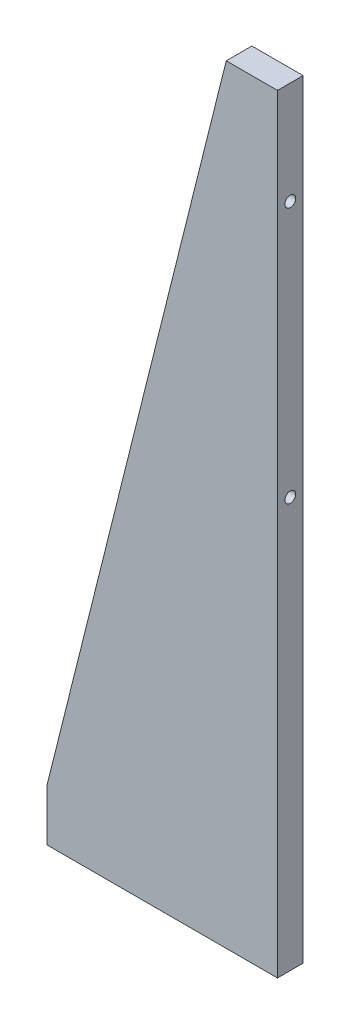
SolidWorks part; units mm, degrees
ref_plane "前视基准面" through (0, 0, 0) normal (0, 0, 1) x (1, 0, 0)
ref_plane "上视基准面" through (0, 0, 0) normal (0, 1, 0) x (1, 0, 0)
ref_plane "右视基准面" through (0, 0, 0) normal (1, 0, 0) x (0, 0, -1)
sketch "草图1" plane through (0, 0, 0) normal (0, 0, 1) x (1, 0, 0)
  line L1 (45, -150) -> (-45, -150)
  line L2 (45, -150) -> (45, 150)
  line L3 (45, 150) -> (-45, 150)
  line L4 (-45, -150) -> (-45, 150)
  line L5 (45, -150) -> (-45, 150) construction
  line L6 (45, 150) -> (-45, -150) construction
  point P0 (0, 0)
  dimension "D1" = 300
  dimension "D2" = 90
extrude "凸台-拉伸1" add sketch "草图1" along normal blind 10
sketch "草图2" plane through (0, 0, 10) normal (0, 0, 1) x (1, 0, 0)
  line L0 (25, 150) -> (-45, 150)
  line L1 (45, 150) -> (-45, 150) construction
  line L2 (-45, 150) -> (-45, -130)
  line L3 (-45, 150) -> (-45, -150) construction
  line L4 (-45, -130) -> (25, 150)
  line L5 (45, -150) -> (45, 150) construction
  line L6 (-45, -150) -> (45, -150) construction
  dimension "D1" = 20
  dimension "D2" = 20
extrude "切除-拉伸1" cut sketch "草图2" against normal up to next
hole_wizard "M5 螺纹孔1" positions "草图3" profile "草图5" tap size "M5" standard "GB"
sketch "草图3" plane through (0, -150, 0) normal (0, -1, 0) x (-1, 0, 0)
  line L0 (-45, -5) -> (-25, -5) construction
  line L1 (-45, -10) -> (-45, 0) construction
  line L2 (-25, -5) -> (25, -5) construction
  line L5 (0, -5) -> (0, 0) construction
  line L6 (45, 0) -> (-45, 0) construction
  point P0 (-25, -5)
  point P2 (25, -5)
  dimension "D1" = 50
sketch "草图5" plane through (25, -150, 5) normal (1, 0, 0) x (0, 0, -1)
  line L0 (0, 0) -> (0, 15.6618)
  line L1 (0, 15.6618) -> (2.1, 14.4)
  line L2 (2.1, 14.4) -> (2.1, 0)
  line L5 (2.1, 0) -> (0, 0)
  line L10 (0, 15.6618) -> (-2.1, 14.4) construction
  line L11 (0, -6.35) -> (0, 107.95) construction
  dimension "螺纹孔钻头直径" = 4.2
  dimension "螺纹孔钻头深度" = 14.4
  dimension "导头角度" = 118
cosmetic thread "孔螺蚊线1" parameters "D1"=12, "D2"=5
cosmetic thread "孔螺蚊线2" parameters "D1"=12, "D2"=5
hole_wizard "M5 螺纹孔2" positions "草图6" profile "草图7" tap size "M5" standard "GB"
sketch "草图6" plane through (45, 0, 0) normal (1, 0, 0) x (0, 0, -1)
  line L0 (-5, 150) -> (-5, 110) construction
  line L1 (-10, 150) -> (0, 150) construction
  line L2 (-5, 110) -> (-5, 10) construction
  point P0 (-5, 110)
  point P2 (-5, 10)
  dimension "D1" = 40
  dimension "D2" = 100
sketch "草图7" plane through (45, 110, 5) normal (0, 1, 0) x (0, 0, -1)
  line L0 (0, 0) -> (0, 15.6618)
  line L1 (0, 15.6618) -> (2.1, 14.4)
  line L2 (2.1, 14.4) -> (2.1, 0)
  line L5 (2.1, 0) -> (0, 0)
  line L10 (0, 15.6618) -> (-2.1, 14.4) construction
  line L11 (0, -6.35) -> (0, 107.95) construction
  dimension "螺纹孔钻头直径" = 4.2
  dimension "螺纹孔钻头深度" = 14.4
  dimension "导头角度" = 118
cosmetic thread "孔螺蚊线3" parameters "D1"=12, "D2"=5
cosmetic thread "孔螺蚊线4" parameters "D1"=12, "D2"=5
